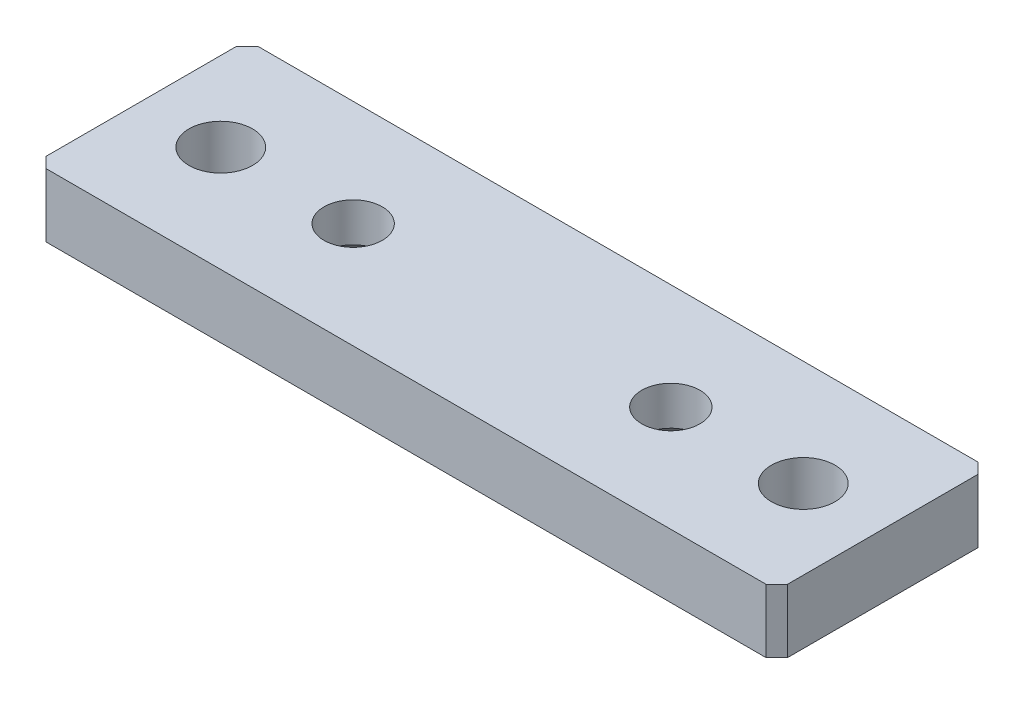
SolidWorks part; units mm, degrees
material "Q235"
ref_plane "Front Plane" through (0, 0, 0) normal (0, 0, 1) x (1, 0, 0)
ref_plane "Top Plane" through (0, 0, 0) normal (0, 1, 0) x (1, 0, 0)
ref_plane "Right Plane" through (0, 0, 0) normal (1, 0, 0) x (0, 0, -1)
sketch "Sketch5" plane through (0, 0, 0) normal (0, 1, 0) x (1, 0, 0)
  line L1 (-70, 20) -> (70, 20)
  line L2 (-70, 20) -> (-70, -20)
  line L3 (-70, -20) -> (70, -20)
  line L4 (70, 20) -> (70, -20)
  line L5 (-70, 20) -> (70, -20) construction
  line L6 (-70, -20) -> (70, 20) construction
  point P0 (0, 0)
  dimension "D1" = 40
  dimension "D2" = 140
extrude "Boss-Extrude1" add sketch "Sketch5" along normal blind 12
hole_wizard "M10 Clearance Hole1" positions "Sketch7" profile "Sketch8" hole size "M10" standard "GB"
sketch "Sketch7" plane through (0, 12, 0) normal (0, 1, 0) x (1, 0, 0)
  line L0 (0, 0) -> (0, 20) construction
  line L1 (70, 20) -> (-70, 20) construction
  line L3 (-70, 0) -> (-55, 0) construction
  line L4 (-70, 20) -> (-70, -20) construction
  point P0 (-55, 0)
  point P2 (55, 0)
  dimension "D1" = 110
sketch "Sketch8" plane through (-55, 12, 0) normal (1, 0, 0) x (0, 0, 1)
  line L0 (0, 0) -> (0, 56.6052)
  line L1 (0, 56.6052) -> (6, 53)
  line L2 (6, 53) -> (6, 0)
  line L5 (6, 0) -> (0, 0)
  line L10 (0, 56.6052) -> (-6, 53) construction
  line L11 (0, -6.35) -> (0, 107.95) construction
  dimension "孔直径" = 12
  dimension "孔深度" = 53
  dimension "导头角度" = 118
hole_wizard "Hole size (%-based) hex socket countersunk screw type2" positions "Sketch11" profile "Sketch12" countersink size "M10" standard "GB"
sketch "Sketch11" plane through (0, 0, 0) normal (0, -1, 0) x (-1, 0, 0)
  line L0 (0, 0) -> (0, 12.1953) construction
  line L2 (0, 0) -> (30, 0) construction
  point P0 (-30, 0)
  point P2 (30, 0)
  dimension "D1" = 60
sketch "Sketch12" plane through (30, 0, 0) normal (1, 0, 0) x (0, 0, -1)
  line L0 (0, 0) -> (0, 56.3047)
  line L1 (0, 56.3047) -> (5.5, 53)
  line L2 (5.5, 53) -> (5.5, 4.65)
  line L3 (5.5, 4.65) -> (10.15, 0)
  line L5 (10.15, 0) -> (0, 0)
  line L6 (-5.5, 4.65) -> (-10.15, 0) construction
  line L10 (0, 56.3047) -> (-5.5, 53) construction
  line L11 (0, -6.35) -> (0, 107.95) construction
  dimension "孔直径" = 11
  dimension "孔深度" = 53
  dimension "近端锥形沉头孔直径" = 20.3
  dimension "近端锥形沉头孔角度" = 90
  dimension "导头角度" = 118
chamfer "Chamfer1" distance 2 angle 45 4 edges at (-70, 6, 20) (-70, 6, -20) (70, 6, -20) (70, 6, 20)
